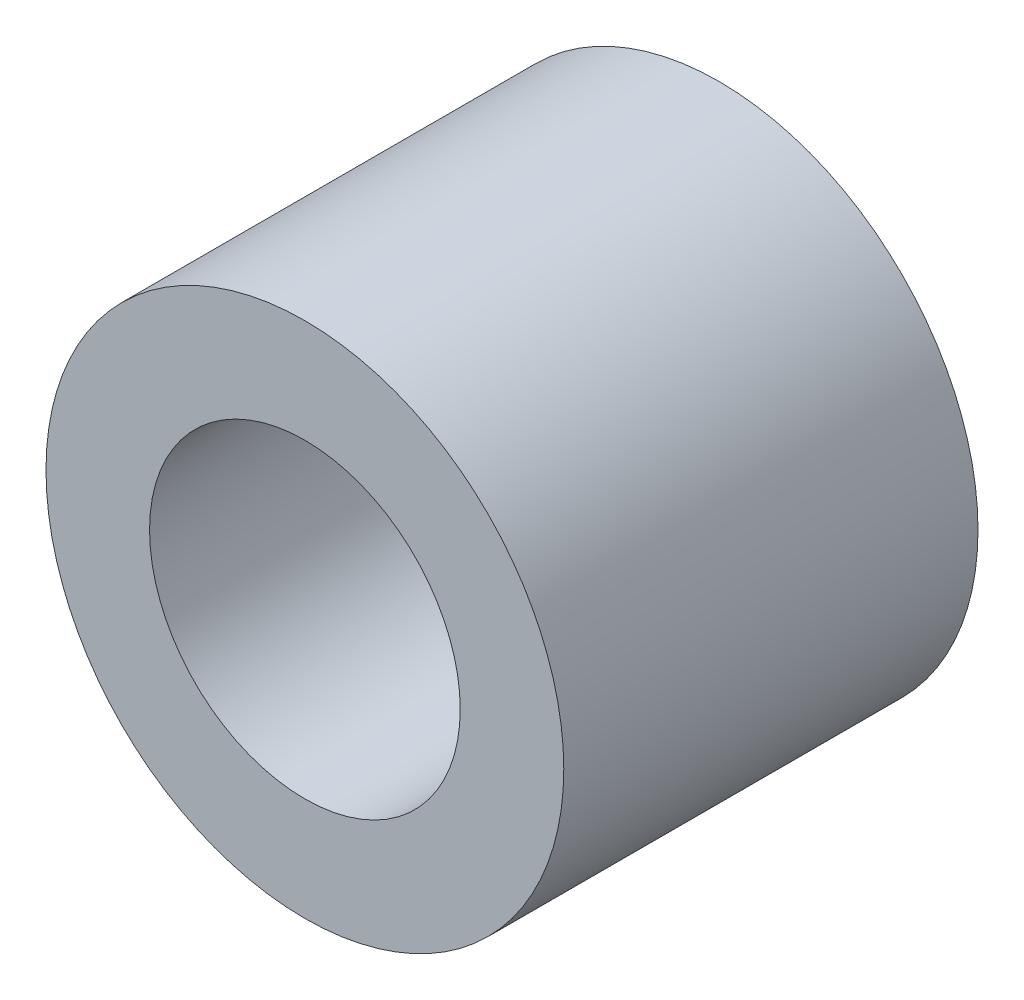
from build123d import *

# Parameters (mm, degrees)
SKETCH1_R           = 25
SKETCH1_R_2         = 15
BOSS_EXTRUDE1_DEPTH = 40


with BuildPart() as part:
    # Sketch1 → Boss-Extrude1 (new body)
    with BuildSketch(Plane.XY):
        Circle(SKETCH1_R)
        Circle(SKETCH1_R_2, mode=Mode.SUBTRACT)
    extrude(amount=BOSS_EXTRUDE1_DEPTH)


solid = part.part
